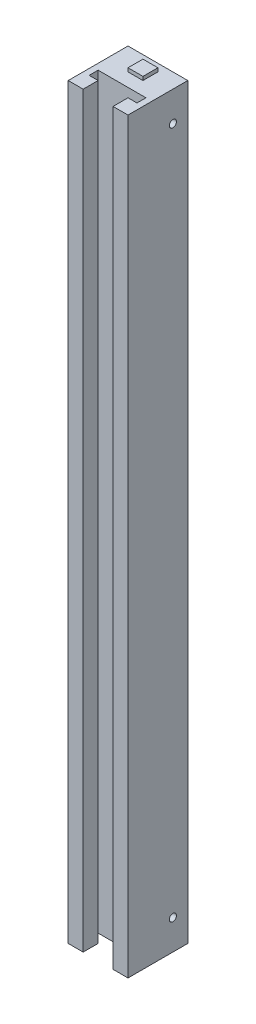
from build123d import *

# Parameters (mm, degrees)
BOSS_EXTRUDE1_DEPTH                    = 250
CBORE_FOR_M2_HEX_CAP_SCREW1_AT_2_COUNT = 2
CBORE_FOR_M2_HEX_CAP_SCREW1_AT_2_PITCH = 230
SKETCH_5_3_W                           = 5
SKETCH_5_3_H                           = 5
BOSS_EXTRUDE2_DEPTH                    = 1.2
SKETCH_5_3_2_W                         = 5
SKETCH_5_3_2_H                         = 5
BOSS_EXTRUDE3_DEPTH                    = 251.2
CUT_EXTRUDE1_START                     = -10
SKETCH6_R                              = 1.2
CUT_EXTRUDE1_DEPTH                     = 10


with BuildPart() as part:
    # Sketch1 → Boss-Extrude1 (new body)
    with BuildSketch(Plane(origin=(0, 0, 0), x_dir=(1, 0, 0), z_dir=(0, 1, 0))):
        Polygon((0, 0), (0, 20), (20, 20), (20, 0), (15, 0), (15, 5), (18, 5), (18, 8), (2, 8), (2, 5), (5, 5), (5, 0), align=None)
    extrude(amount=BOSS_EXTRUDE1_DEPTH)

    # Sketch4 → CBORE for M2 Hex Cap Screw1 (revolve, cut)
    with BuildSketch(Plane(origin=(0, 10, -15), x_dir=(0, 0, 1), z_dir=(0, 1, 0))):
        Polygon((0, 0), (0, 25.721032743), (1.2, 25), (1.2, 1.4), (3.8095, 1.4), (3.8095, 0.025), (3.8345, 0), align=None)
    cbore_for_m2_hex_cap_screw1 = revolve(axis=Axis((-6.35, 10, -15), (1, 0, 0)), mode=Mode.SUBTRACT)

    # CBORE for M2 Hex Cap Screw1 at 2: CBORE for M2 Hex Cap Screw1 ×2
    with Locations(*[(0, i * CBORE_FOR_M2_HEX_CAP_SCREW1_AT_2_PITCH, 0) for i in range(1, CBORE_FOR_M2_HEX_CAP_SCREW1_AT_2_COUNT)]):
        add(cbore_for_m2_hex_cap_screw1, mode=Mode.SUBTRACT)

    # Sketch 5_3 → Boss-Extrude2 (add)
    with BuildSketch(Plane(origin=(0, 250, 0), x_dir=(1, 0, 0), z_dir=(0, 1, 0))):
        with Locations((10, 15)):
            Rectangle(SKETCH_5_3_W, SKETCH_5_3_H)
    extrude(amount=BOSS_EXTRUDE2_DEPTH)

    # Sketch 5_3 2 → Boss-Extrude3 (add)
    with BuildSketch(Plane(origin=(0, 250, 0), x_dir=(1, 0, 0), z_dir=(0, 1, 0))):
        with Locations((10, 15)):
            Rectangle(SKETCH_5_3_2_W, SKETCH_5_3_2_H)
    extrude(amount=-BOSS_EXTRUDE3_DEPTH)

    # Sketch6 → Cut-Extrude1 (cut)
    with BuildSketch(Plane(origin=(12.5, 0, 0), x_dir=(0, 0, -1), z_dir=(1, 0, 0)).offset(CUT_EXTRUDE1_START)):
        with Locations(Location((15, 240, 0), (0, 0, 180))):
            Circle(SKETCH6_R)
        with Locations(Location((15, 10, 0), (0, 0, 180))):
            Circle(SKETCH6_R)
    extrude(amount=CUT_EXTRUDE1_DEPTH, mode=Mode.SUBTRACT)


solid = part.part
